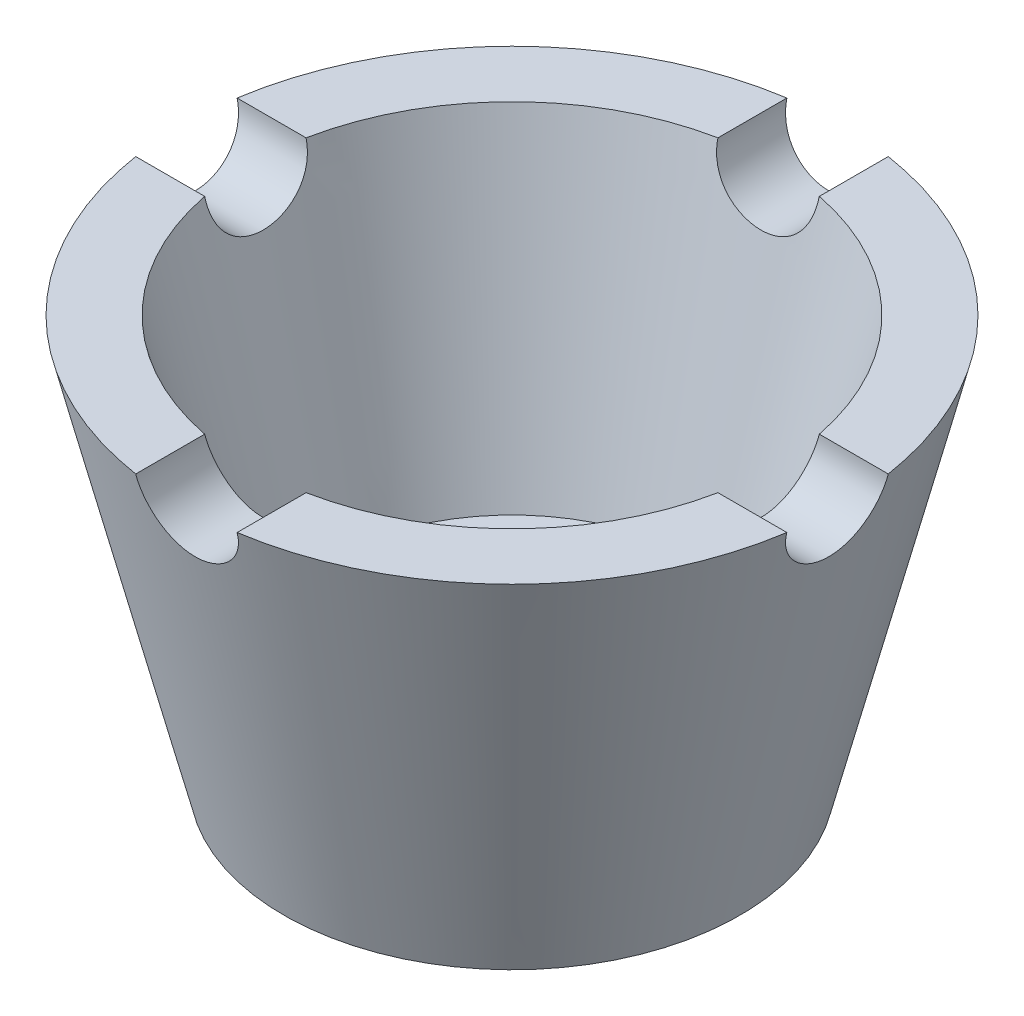
SolidWorks part; units mm, degrees
material "Brass"
ref_plane "Front Plane" through (0, 0, 0) normal (0, 0, 1) x (1, 0, 0)
ref_plane "Top Plane" through (0, 0, 0) normal (0, 1, 0) x (1, 0, 0)
ref_plane "Right Plane" through (0, 0, 0) normal (1, 0, 0) x (0, 0, -1)
sketch "Sketch1" plane through (0, 0, 0) normal (0, 0, 1) x (1, 0, 0)
  line L0 (0, 20) -> (0, -20) construction
  line L1 (32.5, 20) -> (22.5, -20)
  line L2 (22.5, -20) -> (0, -20)
  line L3 (0, -20) -> (0, -10)
  line L4 (25.8, 20) -> (18.3, -10)
  line L5 (0, -10) -> (18.3, -10)
  line L6 (26.1941, 21.5765) -> (16.1941, -18.4235) construction
  line L7 (32.5, 20) -> (25.8, 20)
  dimension "D1" = 40
  dimension "D2" = 32.5
  dimension "D3" = 22.5
  dimension "D5" = 10
  dimension "D4" = 6.5
revolve "Revolve1" add sketch "Sketch1" angle 360 about L0
sketch "Sketch2" plane through (0, -10, 0) normal (0, 1, 0) x (1, 0, 0)
  circle A0 centre (0, 0) radius 12.5
  dimension "D1" = 25
extrude "Cut-Extrude1" cut sketch "Sketch2" against normal blind 10
sketch "Sketch4" plane through (0, 0, 0) normal (0, 0, 1) x (1, 0, 0)
  line L0 (25.8, 20) -> (-25.8, 20) construction
  line L1 (-5, 20) -> (5, 20)
  arc A0 (-5, 20) -> (5, 20) centre (0, 20) ccw
  dimension "D1" = 10
extrude "Cut-Extrude2" cut sketch "Sketch4" against normal mid plane 80
pattern_circular "CirPattern1" count 4 over 360 about axis through (0, -20, 0) along (0, 1, 0) of "Cut-Extrude2"
